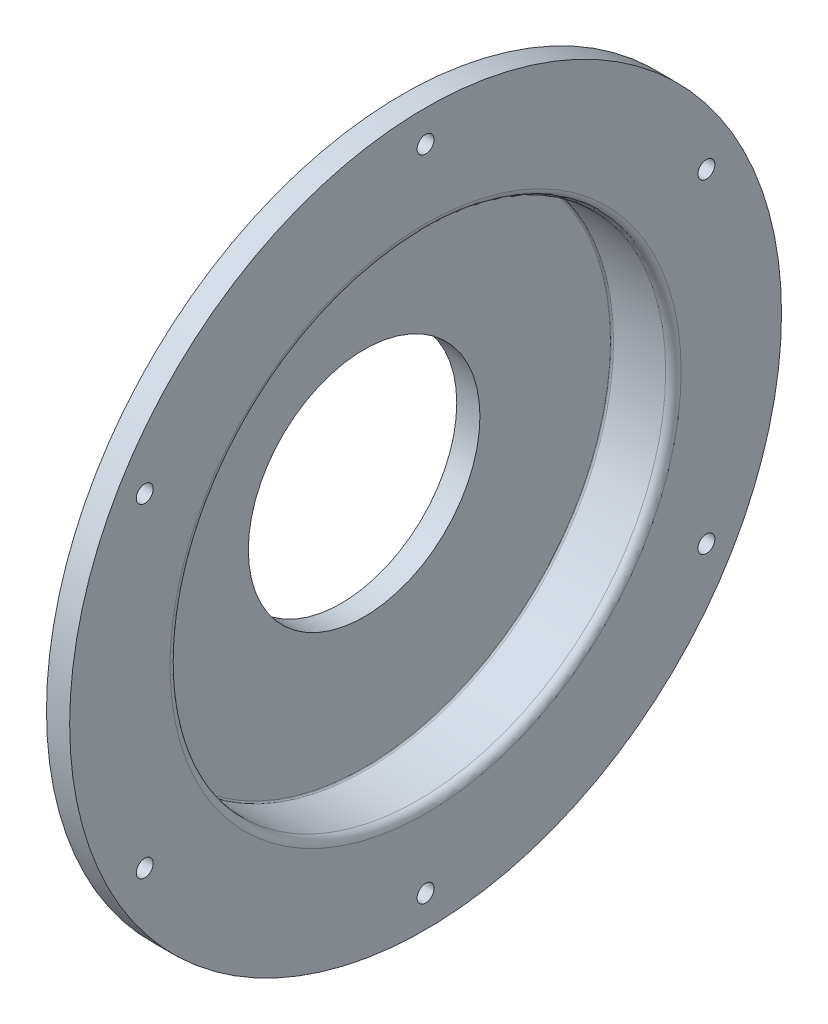
from build123d import *

# Parameters (mm, degrees)
SKETCH2_R          = 5.5
CUT_EXTRUDE1_DEPTH = 85


with BuildPart() as part:
    # Sketch1 → Revolve1 (revolve)
    with BuildSketch(Plane.XY, mode=Mode.PRIVATE) as revolve1_sk:
        with BuildLine():
            Line((-357.644251927, 160.5), (-391.444251927, 160.5))
            ThreePointArc((-391.444251927, 160.5), (-392.151358708, 160.207106781), (-392.444251927, 159.5))
            Line((-392.444251927, 159.5), (-392.444251927, 131))
            Line((-392.444251927, 131), (-392.444251927, 75))
            Line((-392.444251927, 75), (-407.444251927, 75))
            Line((-407.444251927, 75), (-407.444251927, 131))
            Line((-407.444251927, 131), (-407.444251927, 170.5))
            ThreePointArc((-407.444251927, 170.5), (-405.979785833, 174.035533906), (-402.444251927, 175.5))
            Line((-402.444251927, 175.5), (-372.644251927, 175.5))
            ThreePointArc((-372.644251927, 175.5), (-369.108718021, 176.964466094), (-367.644251927, 180.5))
            Line((-367.644251927, 180.5), (-367.644251927, 205))
            Line((-367.644251927, 205), (-367.644251927, 230.5))
            Line((-367.644251927, 230.5), (-352.644251927, 230.5))
            Line((-352.644251927, 230.5), (-352.644251927, 205.5))
            Line((-352.644251927, 205.5), (-352.644251927, 165.5))
            ThreePointArc((-352.644251927, 165.5), (-354.108718021, 161.964466094), (-357.644251927, 160.5))
        make_face()
    revolve(revolve1_sk.sketch.rotate(Axis((0, 0, 0), (-1, 0, 0)), 90), axis=Axis((0, 0, 0), (-1, 0, 0)))

    # Sketch2 → Cut-Extrude1 (cut)
    with BuildSketch(Plane.ZY.offset(367.644251927)):
        with Locations((0, 210)):
            Circle(SKETCH2_R)
        with Locations((181.865334795, 105)):
            Circle(SKETCH2_R)
        with Locations((181.865334795, -105)):
            Circle(SKETCH2_R)
        with Locations((0, -210)):
            Circle(SKETCH2_R)
        with Locations((-181.865334795, -105)):
            Circle(SKETCH2_R)
        with Locations((-181.865334795, 105)):
            Circle(SKETCH2_R)
    extrude(amount=-CUT_EXTRUDE1_DEPTH, mode=Mode.SUBTRACT)


solid = part.part
